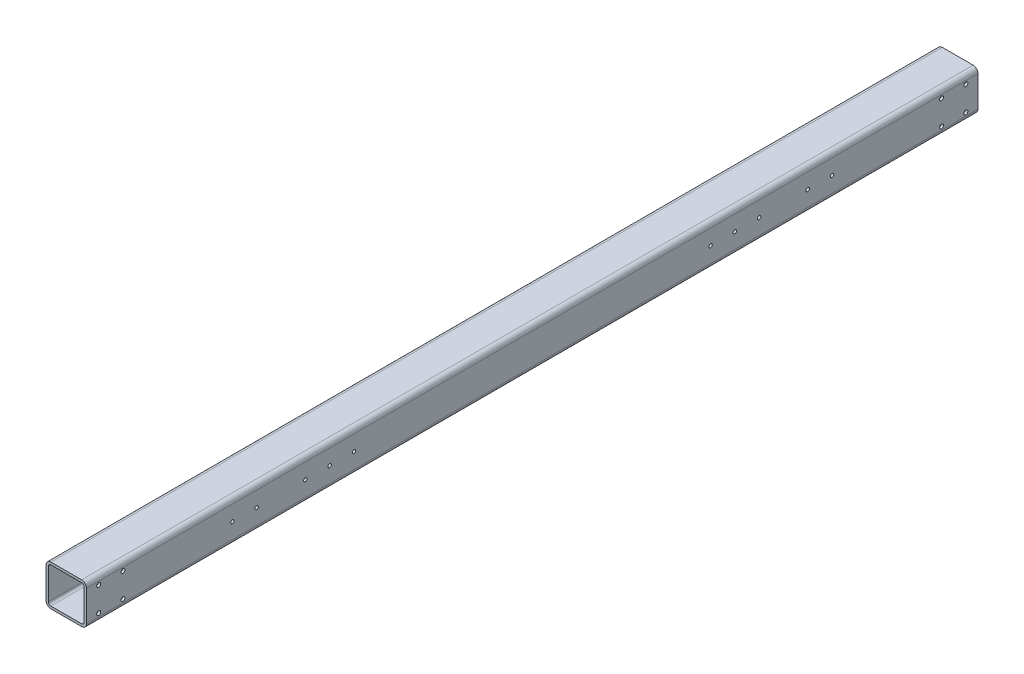
SolidWorks part; units mm, degrees
ref_plane "前视基准面" through (0, 0, 0) normal (0, 0, 1) x (1, 0, 0)
ref_plane "上视基准面" through (0, 0, 0) normal (0, 1, 0) x (1, 0, 0)
ref_plane "右视基准面" through (0, 0, 0) normal (1, 0, 0) x (0, 0, -1)
sketch "草图1" plane through (0, 0, 0) normal (0, 1, 0) x (1, 0, 0)
  line L0 (0, 0) -> (0, 1100)
  dimension "D1" = 1100
other "Gb／6728-1986方形空心型钢 050 X 50 X 3(1)"
ref_plane "基准面1" through (0, 0, 0) normal (0, 0, -1) x (-1, 0, 0)
sketch "Sketch1" plane through (0, 0, 0) normal (0, 0, -1) x (-1, 0, 0)
  line L0 (-19, -22) -> (19, -22)
  line L1 (-22, -19) -> (-22, 19)
  line L2 (19, 22) -> (-19, 22)
  line L3 (22, 19) -> (22, -19)
  line L4 (-19, -25) -> (19, -25)
  line L5 (-25, -19) -> (-25, 19)
  line L6 (19, 25) -> (-19, 25)
  line L7 (25, 19) -> (25, -19)
  arc A0 (25, 19) -> (19, 25) centre (19, 19) ccw
  arc A1 (19, -25) -> (25, -19) centre (19, -19) ccw
  arc A2 (-25, -19) -> (-19, -25) centre (-19, -19) ccw
  arc A3 (-19, 25) -> (-25, 19) centre (-19, 19) ccw
  arc A4 (-19, 22) -> (-22, 19) centre (-19, 19) ccw
  arc A5 (22, 19) -> (19, 22) centre (19, 19) ccw
  arc A6 (19, -22) -> (22, -19) centre (19, -19) ccw
  arc A7 (-22, -19) -> (-19, -22) centre (-19, -19) ccw
  point P0 (-25, 0)
  point P1 (25, 0)
  point P2 (0, 25)
  point P3 (0, -25)
  point P4 (0, 0)
  point P5 (-25, -25)
  point P6 (25, -25)
  point P7 (25, 25)
  point P8 (-25, 25)
  point P33 (0, 0)
  dimension "D1" = 6
  dimension "Thickness" = 3
  dimension "V_leg" = 50
hole_wizard "M5 螺纹孔1" positions "草图2" profile "草图3" tap size "M5" standard "GB"
sketch "草图2" plane through (25, 0, 0) normal (1, 0, 0) x (0, 0, -1)
  point P0 (180, 0)
  point P2 (210, 0)
sketch "草图3" plane through (25, 0, -180) normal (0, 1, 0) x (0, 0, -1)
  line L0 (0, 0) -> (0, 13.6618)
  line L1 (0, 13.6618) -> (2.1, 12.4)
  line L2 (2.1, 12.4) -> (2.1, 0)
  line L5 (2.1, 0) -> (0, 0)
  line L10 (0, 13.6618) -> (-2.1, 12.4) construction
  line L11 (0, -6.35) -> (0, 107.95) construction
  dimension "螺纹孔钻头直径" = 4.2
  dimension "螺纹孔钻头深度" = 12.4
  dimension "导头角度" = 118
cosmetic thread "孔螺蚊线1" parameters "D1"=3, "D2"=5
cosmetic thread "孔螺蚊线2" parameters "D1"=3, "D2"=5
hole_wizard "M5 螺纹孔2" positions "草图4" profile "草图5" tap size "M5" standard "GB"
sketch "草图4" plane through (25, 0, 0) normal (1, 0, 0) x (0, 0, -1)
  point P0 (270, 0)
  point P3 (300, 0)
  point P6 (330, 0)
sketch "草图5" plane through (25, 0, -270) normal (0, 1, 0) x (0, 0, -1)
  line L0 (0, 0) -> (0, 16.2618)
  line L1 (0, 16.2618) -> (2.1, 15)
  line L2 (2.1, 15) -> (2.1, 0)
  line L5 (2.1, 0) -> (0, 0)
  line L10 (0, 16.2618) -> (-2.1, 15) construction
  line L11 (0, -6.35) -> (0, 107.95) construction
  dimension "螺纹孔钻头直径" = 4.2
  dimension "螺纹孔钻头深度" = 15
  dimension "导头角度" = 118
cosmetic thread "孔螺蚊线3" parameters "D1"=3, "D2"=5
cosmetic thread "孔螺蚊线4" parameters "D1"=3, "D2"=5
cosmetic thread "孔螺蚊线5" parameters "D1"=3, "D2"=5
hole_wizard "M5 螺纹孔3" positions "草图6" profile "草图7" tap size "M5" standard "GB"
sketch "草图6" plane through (25, 0, 0) normal (1, 0, 0) x (0, 0, -1)
  line L0 (1100, 25) -> (0, 25) construction
  line L1 (1100, 19) -> (1100, -19) construction
  point P0 (920, 0)
  point P2 (890, 0)
  point P4 (830, 0)
  point P6 (800, 0)
  point P8 (770, 0)
  dimension "D1" = 25
  dimension "D2" = 180
  dimension "D3" = 30
  dimension "D4" = 60
  dimension "D5" = 30
  dimension "D6" = 30
sketch "草图7" plane through (25, 0, -920) normal (0, 1, 0) x (0, 0, -1)
  line L0 (0, 0) -> (0, 13.6618)
  line L1 (0, 13.6618) -> (2.1, 12.4)
  line L2 (2.1, 12.4) -> (2.1, 0)
  line L5 (2.1, 0) -> (0, 0)
  line L10 (0, 13.6618) -> (-2.1, 12.4) construction
  line L11 (0, -6.35) -> (0, 107.95) construction
  dimension "螺纹孔钻头直径" = 4.2
  dimension "螺纹孔钻头深度" = 12.4
  dimension "导头角度" = 118
cosmetic thread "孔螺蚊线6" parameters "D1"=3, "D2"=5
cosmetic thread "孔螺蚊线7" parameters "D1"=3, "D2"=5
cosmetic thread "孔螺蚊线8" parameters "D1"=3, "D2"=5
cosmetic thread "孔螺蚊线9" parameters "D1"=3, "D2"=5
cosmetic thread "孔螺蚊线10" parameters "D1"=3, "D2"=5
hole_wizard "M6 螺纹孔1" positions "草图8" profile "草图9" tap size "M6" standard "GB"
sketch "草图8" plane through (25, 0, 0) normal (1, 0, 0) x (0, 0, -1)
  point P0 (15, 15)
  point P3 (45, 15)
  point P6 (15, -15)
  point P9 (45, -15)
  point P12 (1055, 15)
  point P15 (1085, 15)
  point P18 (1055, -15)
  point P21 (1085, -15)
sketch "草图9" plane through (25, 15, -15) normal (0, 1, 0) x (0, 0, -1)
  line L0 (0, 0) -> (0, 16.5022)
  line L1 (0, 16.5022) -> (2.5, 15)
  line L2 (2.5, 15) -> (2.5, 0)
  line L5 (2.5, 0) -> (0, 0)
  line L10 (0, 16.5022) -> (-2.5, 15) construction
  line L11 (0, -6.35) -> (0, 107.95) construction
  dimension "螺纹孔钻头直径" = 5
  dimension "螺纹孔钻头深度" = 15
  dimension "导头角度" = 118
cosmetic thread "孔螺蚊线11" parameters "D1"=3, "D2"=6
cosmetic thread "孔螺蚊线12" parameters "D1"=3, "D2"=6
cosmetic thread "孔螺蚊线13" parameters "D1"=3, "D2"=6
cosmetic thread "孔螺蚊线14" parameters "D1"=3, "D2"=6
cosmetic thread "孔螺蚊线15" parameters "D1"=3, "D2"=6
cosmetic thread "孔螺蚊线16" parameters "D1"=3, "D2"=6
cosmetic thread "孔螺蚊线17" parameters "D1"=3, "D2"=6
cosmetic thread "孔螺蚊线18" parameters "D1"=3, "D2"=6
